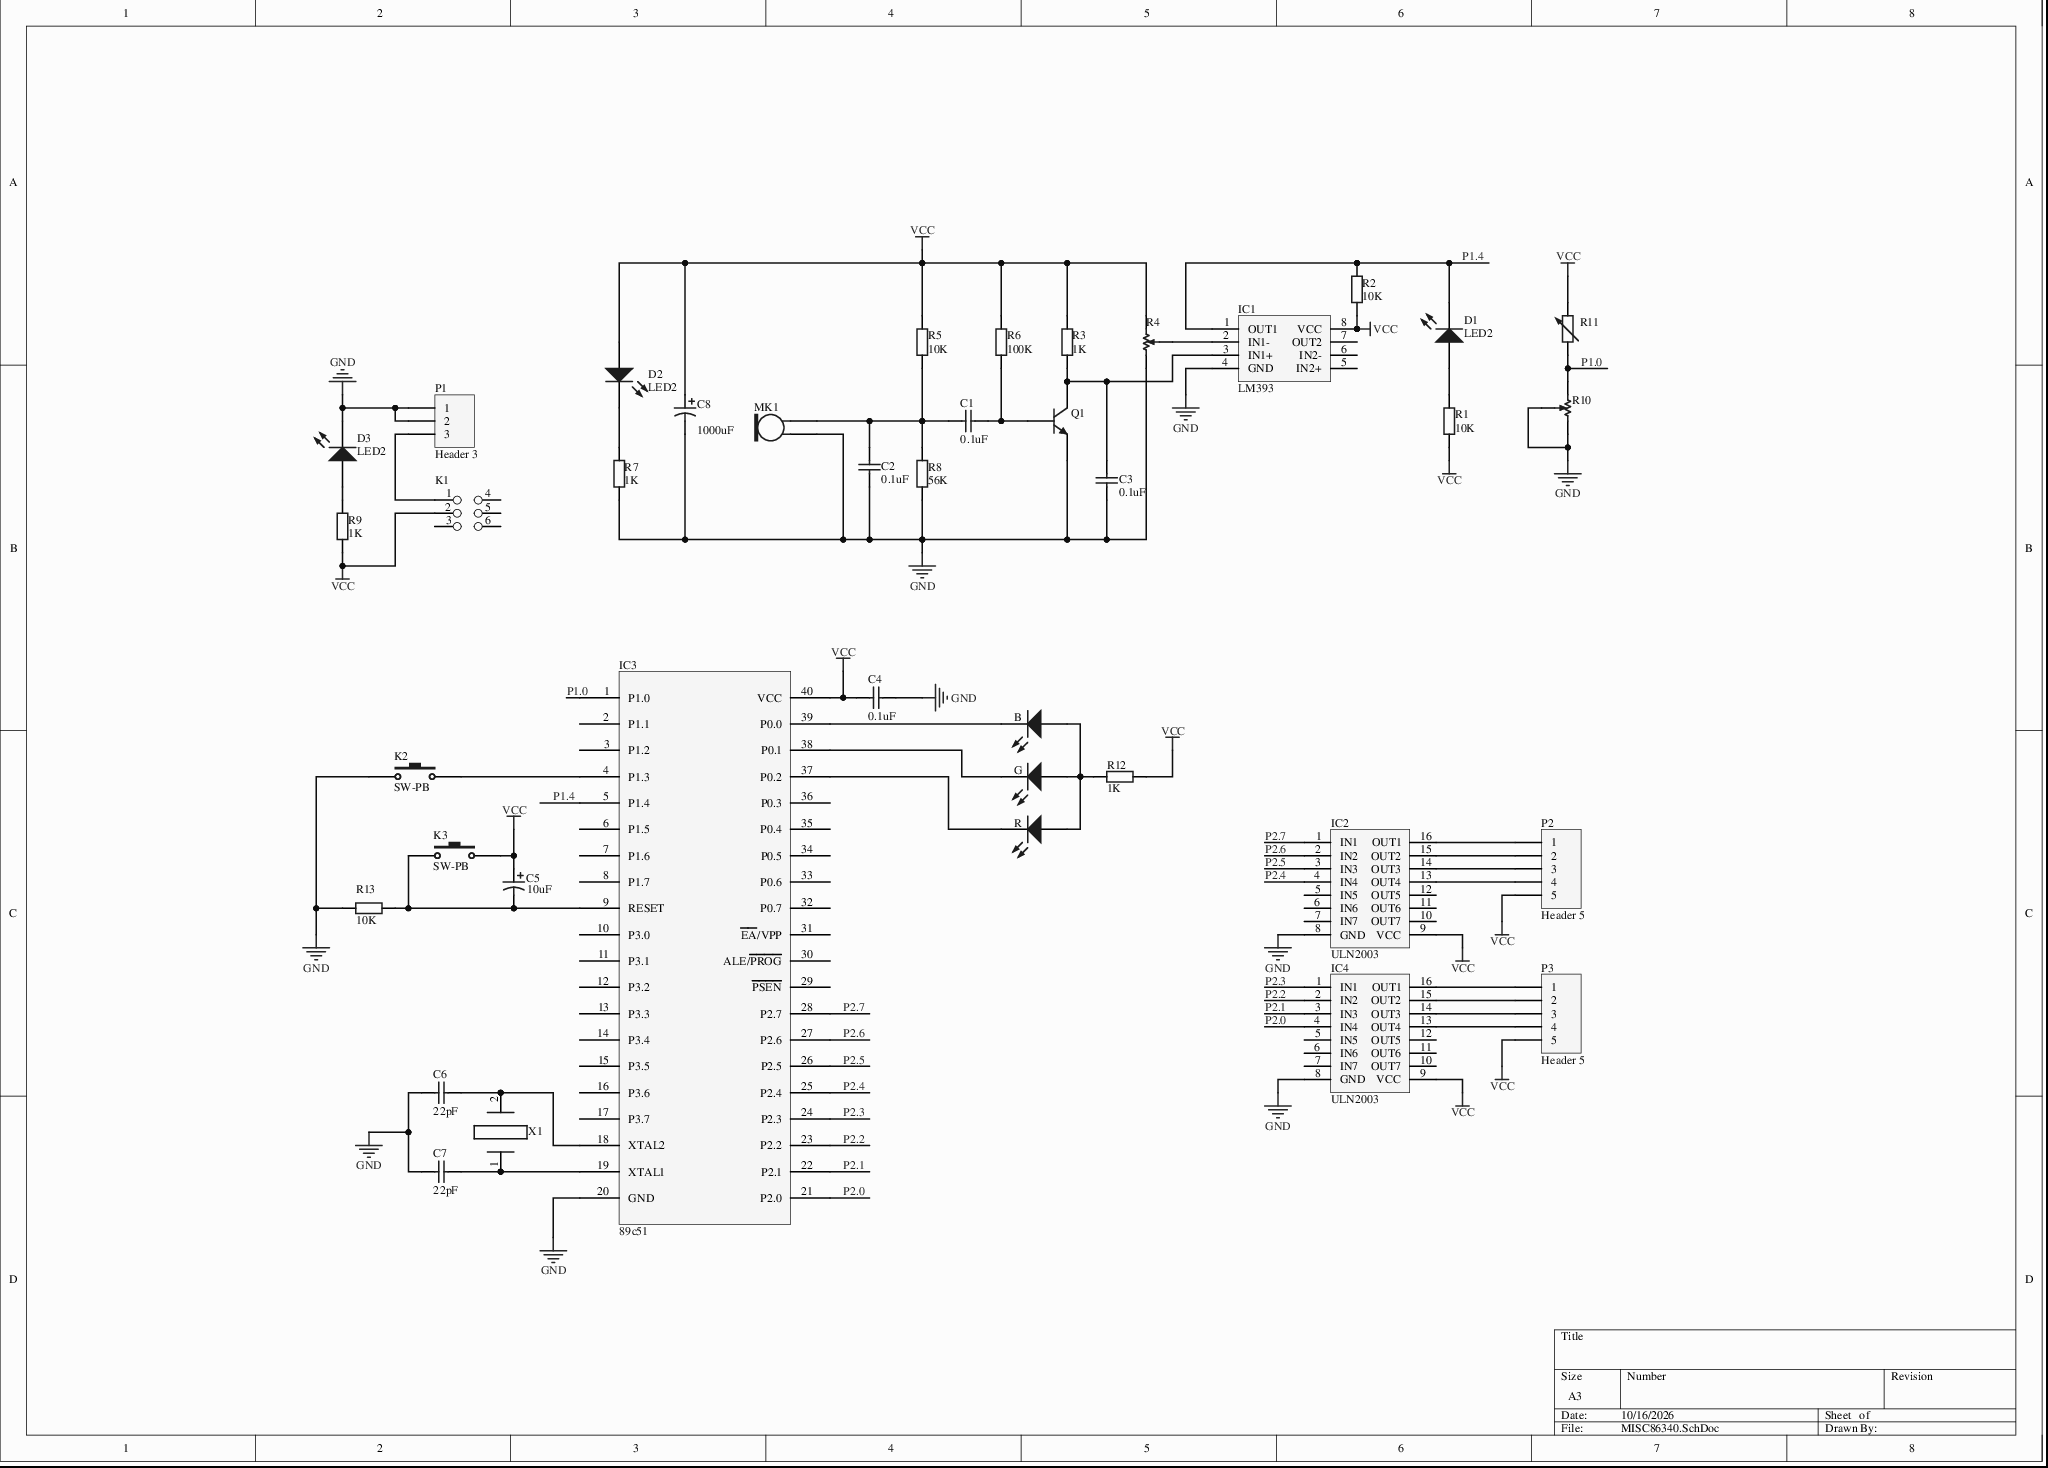
[diagram p0: MISC86340.SchDoc]
# Altium project MISC86340.PrjPcb
1 sheet, 40 parts. Net scope: global (net labels, ports and power ports of the same name join across sheets).
Board file: MISC86340.PcbDoc

## Sheet MISC86340.SchDoc
size A3

### Parts
B  LED2  [3.2X1.6X1.1]  (value not drawn)
C1  value 0.1uF  [RAD-0.3]  (hidden comment: Cap)
C2  value 0.1uF  [RAD-0.3]  (hidden comment: Cap)
C3  value 0.1uF  [RAD-0.3]  (hidden comment: Cap)
C4  value 0.1uF  [RAD-0.3]  (hidden comment: Cap)
C5  value 10uF  [RB7.6-15]  (hidden comment: Cap Pol1)
C6  value 22pF  [RAD-0.3]  (hidden comment: Cap)
C7  value 22pF  [RAD-0.3]  (hidden comment: Cap)
C8  value 1000uF  [RB7.6-15]  (hidden comment: Cap Pol1)
D1  LED2  [3.2X1.6X1.1]
D2  LED2  [3.2X1.6X1.1]
D3  LED2  [3.2X1.6X1.1]
G  LED2  [3.2X1.6X1.1]  (value not drawn)
IC1  LM393  [LM393]
IC2  ULN2003  [ULN2003]
IC3  89c51  [89c51]
IC4  ULN2003  [ULN2003]
K1  Component_1  [自锁开关]  (value not drawn)
K2  SW-PB  [SPST-2]
K3  SW-PB  [SPST-2]
MK1  Mic2  [PIN2]  (value not drawn)
P1  Header 3  [HDR1X3]
P2  Header 5  [HDR1X5]
P3  Header 5  [HDR1X5]
Q1  2N3904  [TO-92A]  (value not drawn)
R  LED2  [3.2X1.6X1.1]  (value not drawn)
R1  value 10K  [AXIAL-0.4]  (hidden comment: Res2)
R2  value 10K  [AXIAL-0.4]  (hidden comment: Res2)
R3  value 1K  [AXIAL-0.4]  (hidden comment: Res2)
R4  RPot SM  [POT4MM-2]  (value not drawn)
R5  value 10K  [AXIAL-0.4]  (hidden comment: Res2)
R6  value 100K  [AXIAL-0.4]  (hidden comment: Res2)
R7  1K  [AXIAL-0.4]
R8  56K  [AXIAL-0.4]
R9  1K  [AXIAL-0.4]
R10  RPot SM  [POT4MM-2]  (value not drawn)
R11  Res Adj2  [AXIAL-0.6]  (value not drawn)
R12  value 1K  [AXIAL-0.4]  (hidden comment: Res2)
R13  value 10K  [AXIAL-0.4]  (hidden comment: Res2)
X1  Component_1  [LC-HC-49S]  (value not drawn)

### Nets
GND: C2.2 C3.2 C4.2 C6.2 C7.2 C8.2 D3.2(K) IC1.4(GND) IC2.8(GND) IC3.20(GND) IC4.8(GND) K2.1 MK1.1 P1.1 P1.2 Q1.1(E) R4.CCW(-) R7.1 R8.1 R10.CW(+) R10.W R13.2
VCC: C4.1 C5.1 C8.1 D2.1(A) IC1.8(VCC) IC2.9(VCC) IC3.40(VCC) IC4.9(VCC) K1.2 K3.2 P2.5 P3.5 R1.1 R2.1 R3.2 R4.CW(+) R5.2 R6.2 R9.1 R11.2 R12.1
P1.0: IC3.1(P1.0) R10.CCW(-) R11.1
P1.4: D1.2(K) IC1.1(OUT1) IC3.5(P1.4) R2.2
P2.0: IC3.21(P2.0) IC4.4(IN4)
P2.1: IC3.22(P2.1) IC4.3(IN3)
P2.2: IC3.23(P2.2) IC4.2(IN2)
P2.3: IC3.24(P2.3) IC4.1(IN1)
P2.4: IC2.4(IN4) IC3.25(P2.4)
P2.5: IC2.3(IN3) IC3.26(P2.5)
P2.6: IC2.2(IN2) IC3.27(P2.6)
P2.7: IC2.1(IN1) IC3.28(P2.7)
NetB_1: B.1(A) G.1(A) R.1(A) R12.2
NetB_2: B.2(K) IC3.39(P0.0)
NetC1_1: C1.1 C2.1 MK1.2 R5.1 R8.2
NetC1_2: C1.2 Q1.2(B) R6.1
NetC3_1: C3.1 IC1.3(IN1+) Q1.3(C) R3.1
NetC5_2: C5.2 IC3.9(RESET) K3.1 R13.1
NetC6_1: C6.1 IC3.18(XTAL2) X1.2
NetC7_1: C7.1 IC3.19(XTAL1) X1.1
NetD1_1: D1.1(A) R1.2
NetD2_2: D2.2(K) R7.2
NetD3_1: D3.1(A) R9.2
NetG_2: G.2(K) IC3.38(P0.1)
NetIC1_2: IC1.2(IN1-) R4.W
NetIC2_13: IC2.13(OUT4) P2.4
NetIC2_14: IC2.14(OUT3) P2.3
NetIC2_15: IC2.15(OUT2) P2.2
NetIC2_16: IC2.16(OUT1) P2.1
NetIC3_4: IC3.4(P1.3) K2.2
NetIC3_37: IC3.37(P0.2) R.2(K)
NetIC4_13: IC4.13(OUT4) P3.4
NetIC4_14: IC4.14(OUT3) P3.3
NetIC4_15: IC4.15(OUT2) P3.2
NetIC4_16: IC4.16(OUT1) P3.1
NetK1_1: K1.1 P1.3

Not connected (* = marked no-connect by the designer): IC1 5(IN2+) 6(IN2-) 7(OUT2); IC2 5(IN5) 6(IN6) 7(IN7) 10(OUT7) 11(OUT6) 12(OUT5); IC3 2(P1.1) 3(P1.2) 6(P1.5) 7(P1.6) 8(P1.7) 10(P3.0) 11(P3.1) 12(P3.2) 13(P3.3) 14(P3.4) 15(P3.5) 16(P3.6) 17(P3.7) 29(~{PSEN}) 30(ALE/~{PROG}) 31(~{EA}/VPP) 32(P0.7) 33(P0.6) 34(P0.5) 35(P0.4) 36(P0.3); IC4 5(IN5) 6(IN6) 7(IN7) 10(OUT7) 11(OUT6) 12(OUT5); K1 3 4 5 6

### Library data of the parts
B D1-D3 G R = LED2: Typical RED, GREEN, YELLOW, AMBER GaAs LED; Published: 8-Jun-2000; LatestRevisionDate: 17-Jul-2002; LatestRevisionNote: Re-released for DXP Platform.; PackageVersion: Feb-2002; PackageReference: 3.2X1.6X1.1; PackageDescription: SM LED; 2 Flat Leads; Publisher: Altium Limited
C1-C4 C6 C7 = Cap: Capacitor; Published: 8-Jun-2000; LatestRevisionDate: 17-Jul-2002; LatestRevisionNote: Re-released for DXP Platform.; PackageReference: RAD-0.3; PackageDescription: Radial Cap, Thru-Hole; 2 Leads; 0.3 in Pin Spacing; Publisher: Altium Limited
C5 C8 = Cap Pol1: Polarized Capacitor (Radial); Published: 8-Jun-2000; LatestRevisionDate: 17-Jul-2002; LatestRevisionNote: Re-released for DXP Platform.; PackageReference: RB7.6-15; PackageDescription: Polarized Capacitor (Radial); 2 Leads; Publisher: Altium Limited
IC1-IC4 = Component_1
K2 K3 = SW-PB: Switch; Published: 24-Mar-1999; LatestRevisionDate: 17-Jul-2002; LatestRevisionNote: Re-released for DXP Platform.; PackageReference: SPST-2; PackageDescription: Switch; 2 Leads; Publisher: Altium Limited
MK1 = Mic2: Microphone; Published: 24-Mar-1999; LatestRevisionDate: 17-Jul-2002; LatestRevisionNote: Re-released for DXP Platform.; PackageReference: PIN2; Publisher: Altium Limited
P1 = Header 3: Header, 3-Pin; LatestRevisionDate: 17-Jul-2002; LatestRevisionNote: Re-released for DXP Platform.; Publisher: Altium Limited
P2 P3 = Header 5: Header, 5-Pin; LatestRevisionDate: 17-Jul-2002; LatestRevisionNote: Re-released for DXP Platform.; Publisher: Altium Limited
Q1 = 2N3904: NPN General Purpose Amplifier; Published: 8-Jun-2000; LatestRevisionDate: 15-Jan-2003; LatestRevisionNote: PCB Footprint 'BCY-W3/D4.7' replaced; DatasheetVersion: 1997; PackageVersion: Sep-1998; PackageReference: TO-92A; PackageDescription: TO, Flat Index; 3 In-Line, Axial Leads; Body Dia. 4.5mm; Leads 0.51 x 0.48 mm (max); ComponentLink1Description: Manufacturer Link; ComponentLink2Description: Datasheet; ComponentLink2URL: http://www.fairchildsemi.com/ds/2N%2F2N3904.pdf; Publisher: Altium Limited
R1-R3 R5-R9 R12 R13 = Res2: Resistor; Published: 8-Jun-2000; LatestRevisionDate: 17-Jul-2002; LatestRevisionNote: Re-released for DXP Platform.; PackageReference: AXIAL-0.4; PackageDescription: Axial Device, Thru-Hole; 2 Leads; 0.4 in Pin Spacing; Publisher: Altium Limited
  R7 R9: Value: 1K
  R8: Value: 56K
R4 R10 = RPot SM: Square Trimming Potentiometer; Published: 17-Dec-2003; DatasheetVersion: Oct-2003; PackageReference: POT4MM-2; PackageDescription: Square Trimming Potentiometer; ComponentLink1Description: Manufacturer Link; ComponentLink1URL: http://bourns.com/2/search.html; Publisher: Altium Limited
R11 = Res Adj2: Variable Resistor; Value: 1K; Set Position: 0.5; Published: 8-Jun-2000; LatestRevisionDate: 17-Jul-2002; LatestRevisionNote: Re-released for DXP Platform.; PackageReference: AXIAL-0.6; PackageDescription: Axial Device, Thru-Hole; 2 Leads; 0.6 in Pin Spacing; Publisher: Altium Limited